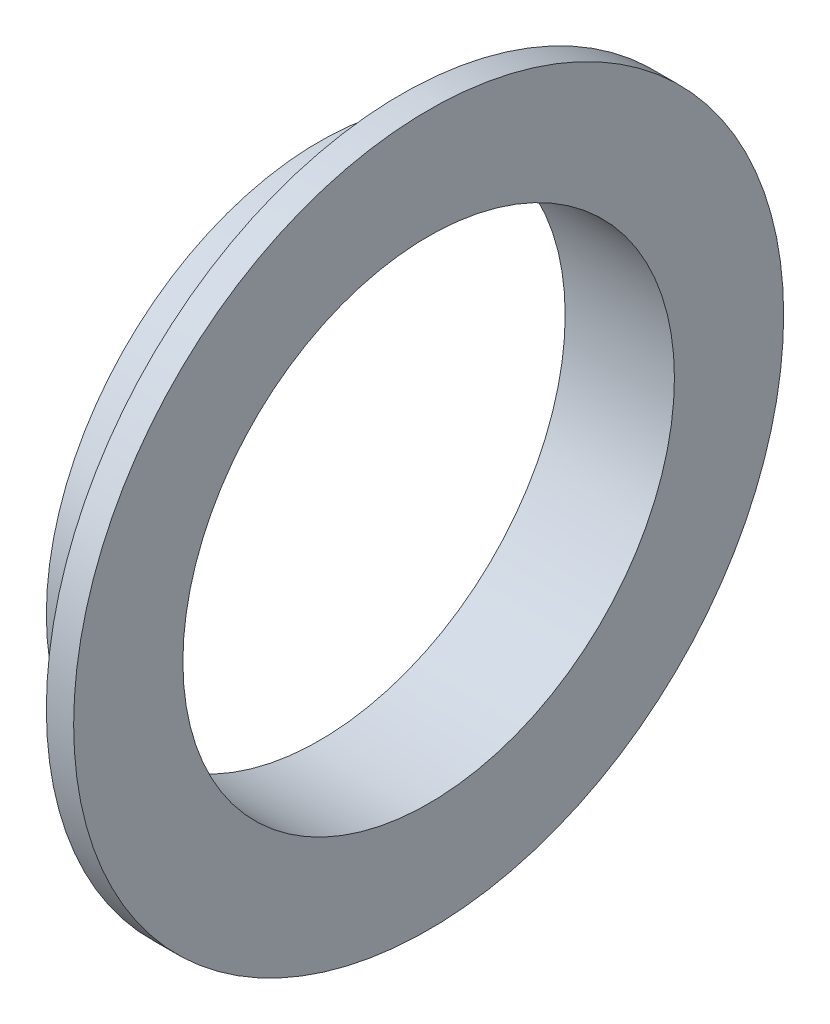
SolidWorks part; units mm, degrees
material "ABS"
ref_plane "前视基准面" through (0, 0, 0) normal (0, 0, 1) x (1, 0, 0)
ref_plane "上视基准面" through (0, 0, 0) normal (0, 1, 0) x (1, 0, 0)
ref_plane "右视基准面" through (0, 0, 0) normal (1, 0, 0) x (0, 0, -1)
other "Configuration Table"
sketch "草图1" plane through (0, 0, 0) normal (0, 1, 0) x (1, 0, 0)
  line L0 (-397.809, 0) -> (19492.643, 0) construction
  line L1 (0, 9) -> (0, 10)
  line L2 (0, 10) -> (3, 10)
  line L3 (3, 10) -> (3, 13)
  line L4 (3, 13) -> (4, 13)
  line L5 (4, 13) -> (4, 9)
  line L6 (4, 9) -> (0, 9)
  dimension "D1" = 18
  dimension "D2" = 20
  dimension "D3" = 4
  dimension "D4" = 26
  dimension "D5" = 1
revolve "旋转1" add sketch "草图1" angle 360 about L0
